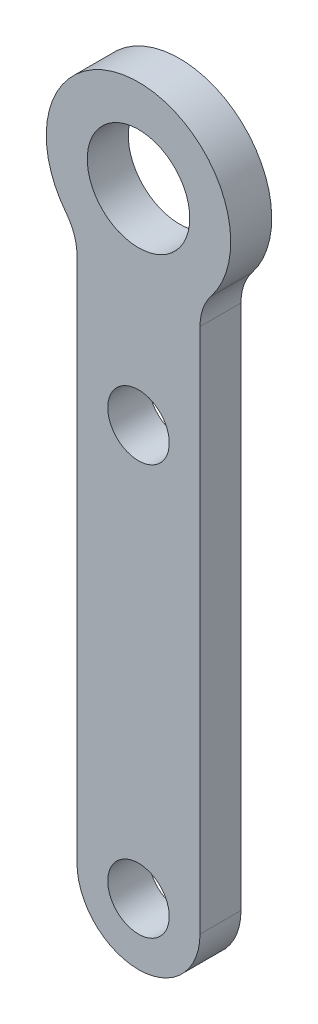
from build123d import *

# Parameters (mm, degrees)
SKETCH1_R           = 5
SKETCH1_R_2         = 3
BOSS_EXTRUDE1_DEPTH = 4


with BuildPart() as part:
    # Sketch1 → Boss-Extrude1 (new body)
    with BuildSketch(Plane.XY):
        with BuildLine():
            Line((-6, -60), (-6, -8.660254038))
            ThreePointArc((-6, -8.660254038), (-6.275444087, -7.023619861), (-7.071428571, -5.567306167))
            ThreePointArc((-7.071428571, -5.567306167), (0, 9), (7.071428571, -5.567306167))
            ThreePointArc((7.071428571, -5.567306167), (6.275444087, -7.023619861), (6, -8.660254038))
            Line((6, -8.660254038), (6, -60))
            ThreePointArc((6, -60), (0, -66), (-6, -60))
        make_face()
        Circle(SKETCH1_R, mode=Mode.SUBTRACT)
        with Locations((0, -20)):
            Circle(SKETCH1_R_2, mode=Mode.SUBTRACT)
        with Locations((0, -60)):
            Circle(SKETCH1_R_2, mode=Mode.SUBTRACT)
    extrude(amount=BOSS_EXTRUDE1_DEPTH)


solid = part.part
